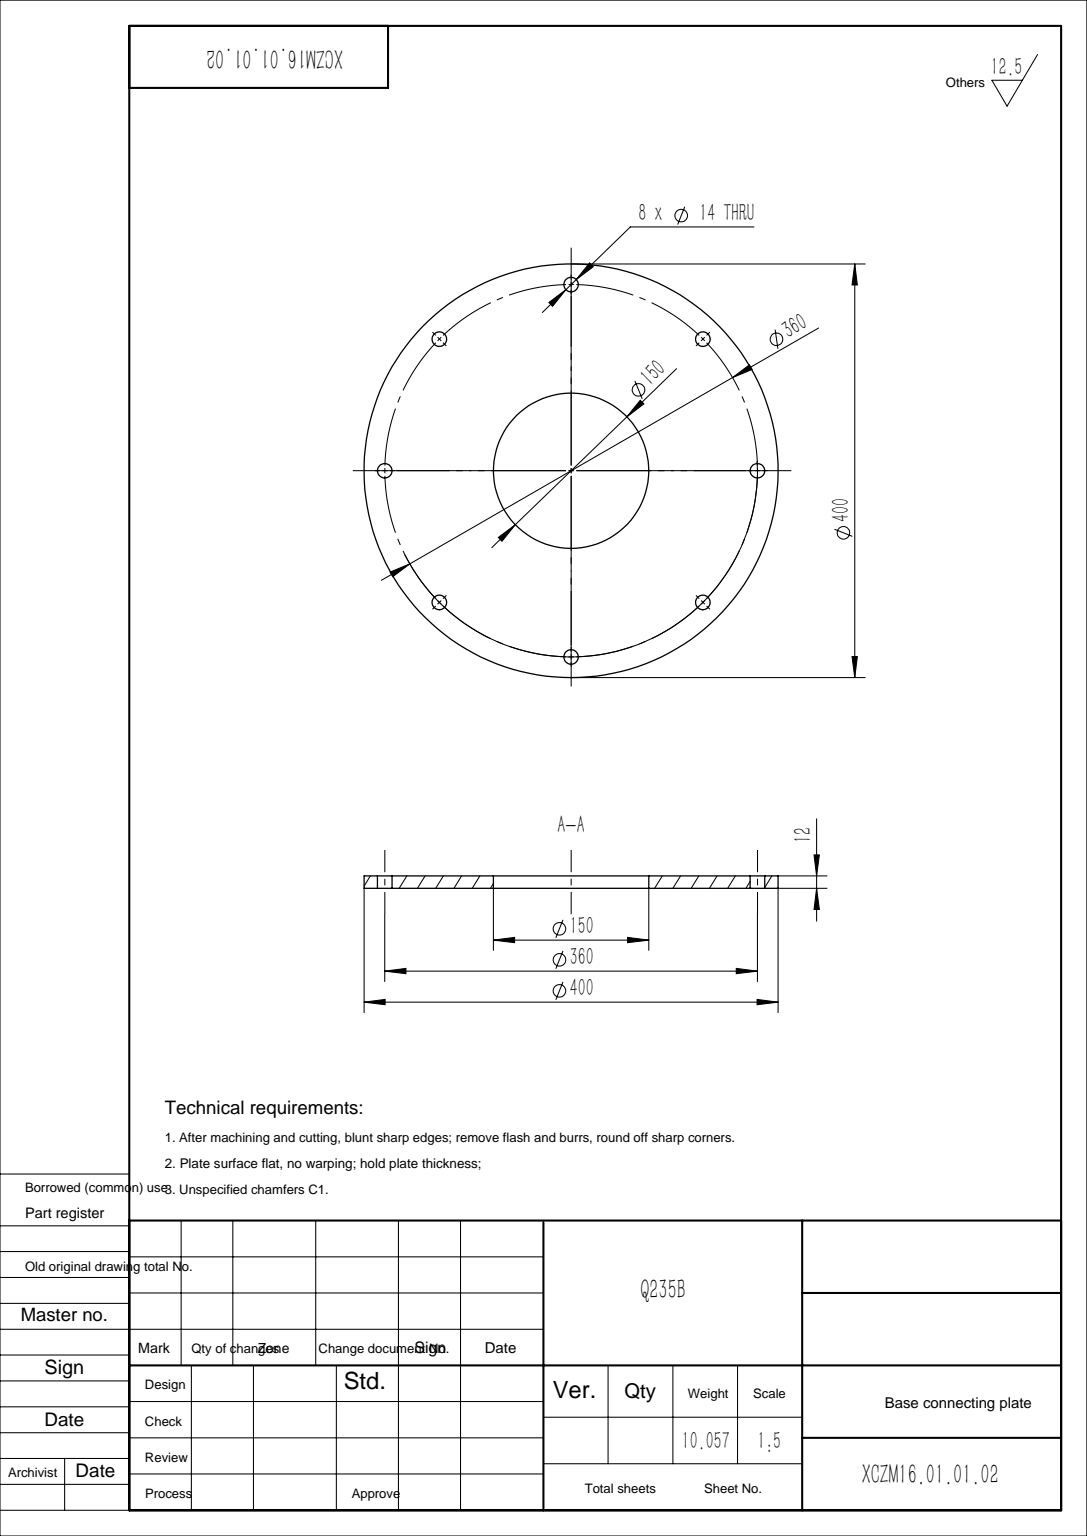
from build123d import *

# Parameters (mm, degrees)
SKETCH1_R                  = 200
SKETCH1_R_2                = 75
BOSS_EXTRUDE1_DEPTH        = 12
F_14_0_14_DIAMETER_HOLE1_D = 14


with BuildPart() as part:
    # Sketch1 → Boss-Extrude1 (new body)
    with BuildSketch(Plane(origin=(0, 0, 0), x_dir=(1, 0, 0), z_dir=(0, 1, 0))):
        with Locations(Location((0, 0, 0), (0, 0, 270))):
            Circle(SKETCH1_R)
        with Locations(Location((0, 0, 0), (0, 0, 270))):
            Circle(SKETCH1_R_2, mode=Mode.SUBTRACT)
    extrude(amount=BOSS_EXTRUDE1_DEPTH)

    # Ø14.0 (14) Diameter Hole1 (through all)
    with Locations(Plane(origin=(0, 12, 0), x_dir=(1, 0, 0), z_dir=(0, 1, 0))):
        with Locations((0, 180), (127.279220614, 127.279220614), (180, 0), (127.279220614, -127.279220614), (0, -180), (-127.279220614, -127.279220614), (-180, 0), (-127.279220614, 127.279220614)):
            Hole(F_14_0_14_DIAMETER_HOLE1_D / 2)


solid = part.part
